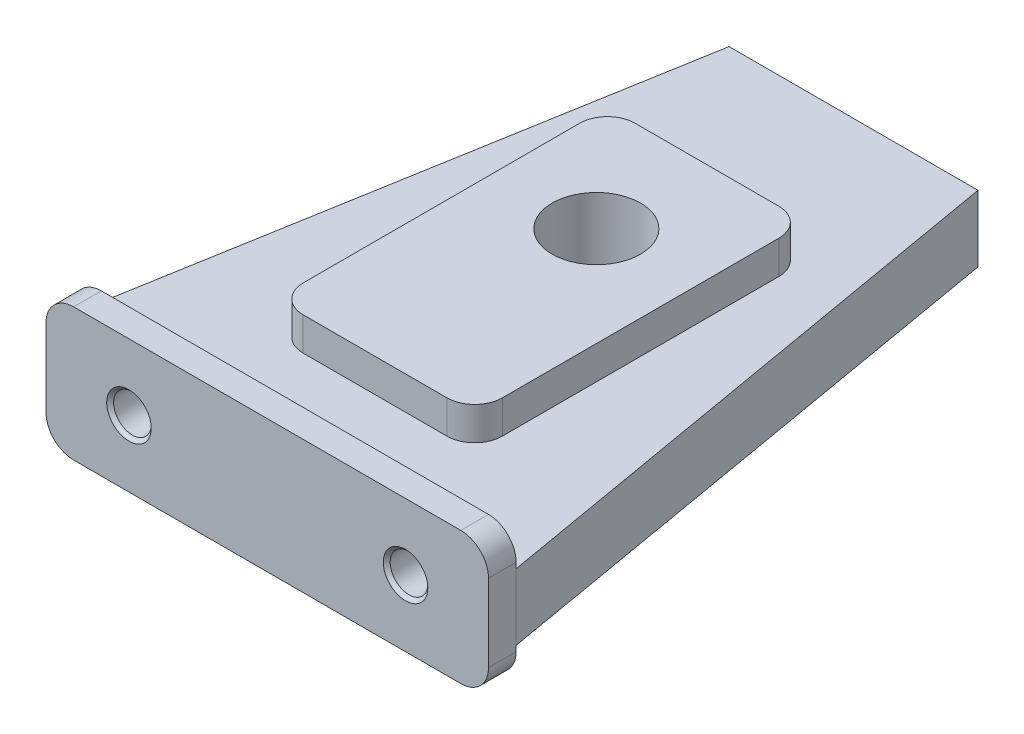
from build123d import *

# Parameters (mm, degrees)
BOSS_EXTRUDE1_DEPTH         = 5
BOSS_EXTRUDE2_DEPTH         = 6
BOSS_EXTRUDE3_DEPTH         = 6
SKETCH4_R                   = 8
CUT_EXTRUDE1_DEPTH          = 21
M8_TAPPED_HOLE1_D           = 6.8
M8_TAPPED_HOLE1_DEPTH       = 20
M8_TAPPED_HOLE1_CSINK_D     = 8.05
M8_TAPPED_HOLE1_CSINK_ANGLE = 90
M8_TAPPED_HOLE1_TIP         = 2.042926105
M6_TAPPED_HOLE1_D           = 5
M6_TAPPED_HOLE1_DEPTH       = 10
M6_TAPPED_HOLE1_CSINK_D     = 6.05
M6_TAPPED_HOLE1_CSINK_ANGLE = 90
M6_TAPPED_HOLE1_TIP         = 1.502151548


with BuildPart() as part:
    # Sketch1 → Boss-Extrude1 (new body)
    with BuildSketch(Plane.XY):
        with BuildLine():
            Line((-35, -12), (35, -12))
            ThreePointArc((35, -12), (38.535533906, -10.535533906), (40, -7))
            Line((40, -7), (40, 7))
            ThreePointArc((40, 7), (38.535533906, 10.535533906), (35, 12))
            Line((35, 12), (-35, 12))
            ThreePointArc((-35, 12), (-38.535533906, 10.535533906), (-40, 7))
            Line((-40, 7), (-40, -7))
            ThreePointArc((-40, -7), (-38.535533906, -10.535533906), (-35, -12))
        make_face()
    extrude(amount=BOSS_EXTRUDE1_DEPTH)

    # Sketch2 → Boss-Extrude2 (add, symmetric)
    with BuildSketch(Plane(origin=(0, 0, 0), x_dir=(1, 0, 0), z_dir=(0, 1, 0))):
        Polygon((-40, 0), (-22.5, 101), (22.5, 101), (40, 0), align=None)
    extrude(amount=BOSS_EXTRUDE2_DEPTH, both=True)

    # Sketch3 → Boss-Extrude3 (add)
    with BuildSketch(Plane(origin=(0, 6, 0), x_dir=(1, 0, 0), z_dir=(0, 1, 0))):
        with BuildLine():
            Line((-13, 14.5), (13, 14.5))
            ThreePointArc((13, 14.5), (16.535533906, 15.964466094), (18, 19.5))
            Line((18, 19.5), (18, 69.5))
            ThreePointArc((18, 69.5), (16.535533906, 73.035533906), (13, 74.5))
            Line((13, 74.5), (-13, 74.5))
            ThreePointArc((-13, 74.5), (-16.535533906, 73.035533906), (-18, 69.5))
            Line((-18, 69.5), (-18, 19.5))
            ThreePointArc((-18, 19.5), (-16.535533906, 15.964466094), (-13, 14.5))
        make_face()
    extrude(amount=BOSS_EXTRUDE3_DEPTH)

    # Sketch4 → Cut-Extrude1 (cut)
    with BuildSketch(Plane(origin=(0, 12, 0), x_dir=(1, 0, 0), z_dir=(0, 1, 0))):
        with Locations(Location((0, 54.5, 0), (0, 0, 270))):
            Circle(SKETCH4_R)
    extrude(amount=-CUT_EXTRUDE1_DEPTH, mode=Mode.SUBTRACT)

    # M8 Tapped Hole1
    with Locations(Plane(origin=(25, 0, 5), x_dir=(1, 0, 0), z_dir=(0, 0, 1))):
        with Locations((0, 0), (-50, 0)):
            CounterSinkHole(M8_TAPPED_HOLE1_D / 2, M8_TAPPED_HOLE1_CSINK_D / 2, depth=M8_TAPPED_HOLE1_DEPTH, counter_sink_angle=M8_TAPPED_HOLE1_CSINK_ANGLE)
            with Locations((0, 0, -(M8_TAPPED_HOLE1_DEPTH + M8_TAPPED_HOLE1_TIP / 2))):  # 118° drill point
                Cone(0, M8_TAPPED_HOLE1_D / 2, M8_TAPPED_HOLE1_TIP, mode=Mode.SUBTRACT)

    # M6 Tapped Hole1
    with Locations(Plane(origin=(14, 0, -101), x_dir=(-1, 0, 0), z_dir=(0, 0, -1))):
        with Locations((0, 0), (28, 0)):
            CounterSinkHole(M6_TAPPED_HOLE1_D / 2, M6_TAPPED_HOLE1_CSINK_D / 2, depth=M6_TAPPED_HOLE1_DEPTH, counter_sink_angle=M6_TAPPED_HOLE1_CSINK_ANGLE)
            with Locations((0, 0, -(M6_TAPPED_HOLE1_DEPTH + M6_TAPPED_HOLE1_TIP / 2))):  # 118° drill point
                Cone(0, M6_TAPPED_HOLE1_D / 2, M6_TAPPED_HOLE1_TIP, mode=Mode.SUBTRACT)


solid = part.part
